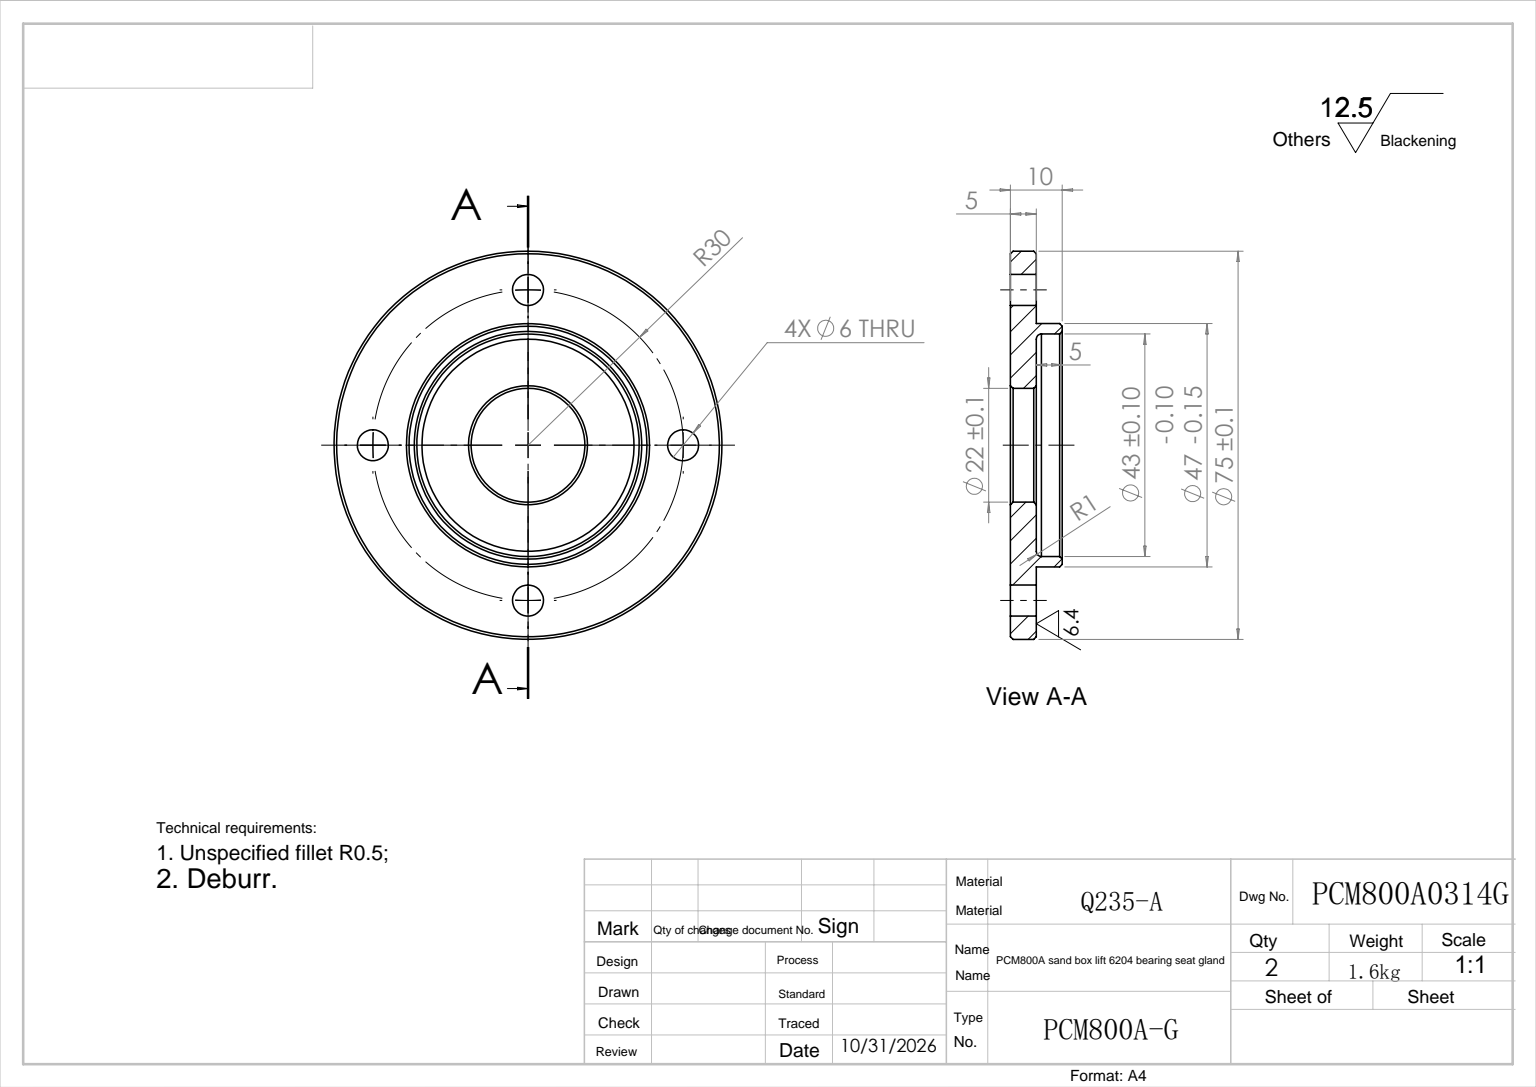
SolidWorks part; units mm, degrees
ref_plane "前视基准面" through (0, 0, 0) normal (0, 0, 1) x (1, 0, 0)
ref_plane "上视基准面" through (0, 0, 0) normal (0, 1, 0) x (1, 0, 0)
ref_plane "右视基准面" through (0, 0, 0) normal (1, 0, 0) x (0, 0, -1)
sketch "草图1" plane through (0, 0, 0) normal (0, 1, 0) x (1, 0, 0)
  circle A0 centre (0, 0) radius 37.5
  circle A1 centre (0, 0) radius 11
extrude "拉伸1" add sketch "草图1" along normal blind 5
sketch "草图2" plane through (0, 0, 0) normal (0, -1, 0) x (1, 0, 0)
  circle A0 centre (0, 0) radius 21.5
  circle A1 centre (0, 0) radius 23.5
  dimension "D1" = 43
  dimension "D2" = 47
extrude "拉伸2" add sketch "草图2" along normal blind 5
sketch "草图3" plane through (0, 5, 0) normal (0, 1, 0) x (-1, 0, 0)
  circle A0 centre (0, 0) radius 30 construction
  circle A1 centre (-30, 0) radius 3
  circle A2 centre (0, 30) radius 3
  circle A3 centre (30, 0) radius 3
  circle A4 centre (0, -30) radius 3
extrude "切除-拉伸1" cut sketch "草图3" against normal through all
chamfer "倒角1" distance 0.5 angle 45 4 edges at (0, 5, 37.5) (0, 0, 37.5) (0, -5, -21.5) (0, -5, -23.5)
fillet "圆角1" radius 1 1 edges at (0, 0, -21.5)
chamfer "倒角2" distance 0.5 angle 45 2 edges at (0, 0, 11) (0, 5, 11)
